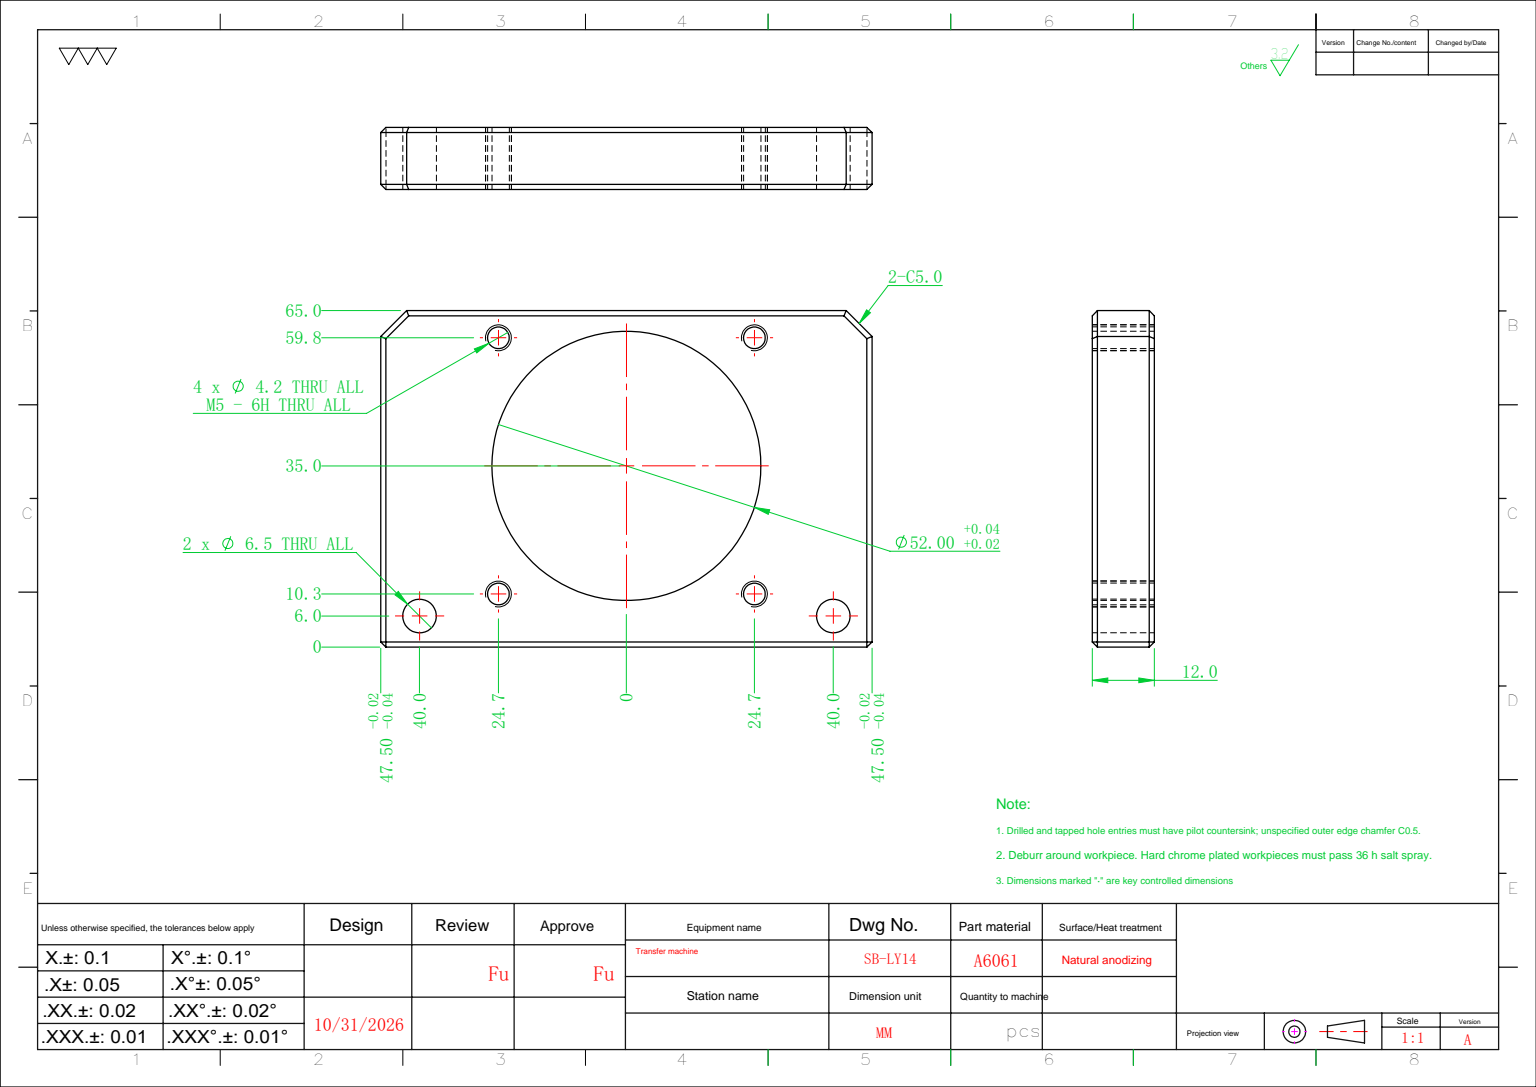
from build123d import *

# Parameters (mm, degrees)
SKETCH_1_W              = 95
SKETCH_1_H              = 65
EXTRUDE_1_DEPTH         = 12
HOLE_WIZARD_6_5_6_5_1_D = 6.5
CHAMFER_1_SIZE          = 5
SKETCH_4_R              = 26
CUT_EXTRUDE_1_DEPTH     = 59.792006259
HOLE_WIZARD_M5_1_D      = 4.2
CHAMFER_2_SIZE          = 1


with BuildPart() as part:
    # 草图1 → 凸台-拉伸1 (new body)
    with BuildSketch(Plane.XY):
        Rectangle(SKETCH_1_W, SKETCH_1_H)
    extrude(amount=EXTRUDE_1_DEPTH)

    # Ø6.5 (6.5) 直径孔1 (through all)
    with Locations(Plane.XY.offset(12)):
        with Locations((-40, -26.5), (40, -26.5)):
            Hole(HOLE_WIZARD_6_5_6_5_1_D / 2)

    # 倒角1
    chamfer_1_edges = [part.edges().sort_by_distance(p)[0] for p in [
        (-47.5, 32.5, 6),
        (47.5, 32.5, 6),
    ]]
    chamfer(chamfer_1_edges, length=CHAMFER_1_SIZE)

    # 草图4 → 切除-拉伸1 (cut, through all)
    with BuildSketch(Plane(origin=(0, 0, 0), x_dir=(-1, 0, 0), z_dir=(0, 0, -1))):
        with Locations((0, 2.5)):
            Circle(SKETCH_4_R)
    extrude(amount=-CUT_EXTRUDE_1_DEPTH, mode=Mode.SUBTRACT)

    # M5 螺纹孔1 (through all)
    with Locations(Plane.XY.offset(12)):
        with Locations((-24.748737342, 27.25), (24.748737342, 27.25), (24.748737342, -22.25), (-24.748737342, -22.25)):
            Hole(HOLE_WIZARD_M5_1_D / 2)

    # 倒角2
    chamfer_2_edges = [part.edges().sort_by_distance(p)[0] for p in [
        (0, -32.5, 12),
        (0, 32.5, 0),
        (0, 32.5, 12),
        (-47.5, -2.5, 0),
        (-45, 30, 0),
        (45, 30, 0),
        (-47.5, -2.5, 12),
        (-45, 30, 12),
        (45, 30, 12),
        (47.5, -2.5, 12),
        (0, -32.5, 0),
        (47.5, -2.5, 0),
        (47.5, -32.5, 6),
        (-47.5, -32.5, 6),
    ]]
    chamfer(chamfer_2_edges, length=CHAMFER_2_SIZE)


solid = part.part
